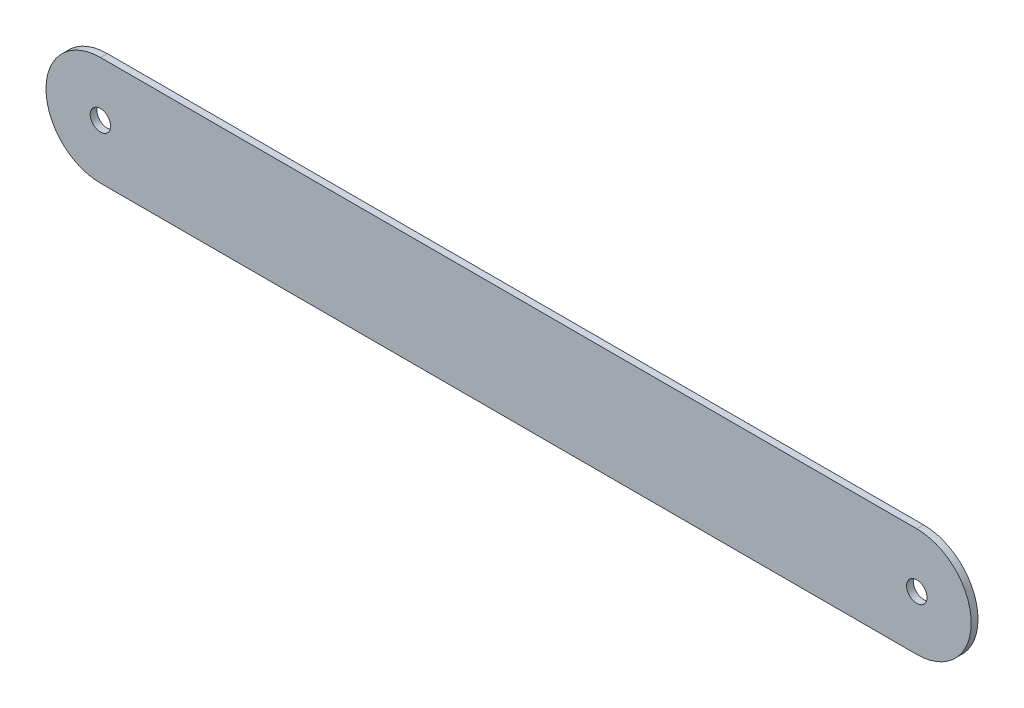
SolidWorks part; units mm, degrees
ref_plane "前视基准面" through (0, 0, 0) normal (0, 0, 1) x (1, 0, 0)
ref_plane "上视基准面" through (0, 0, 0) normal (0, 1, 0) x (1, 0, 0)
ref_plane "右视基准面" through (0, 0, 0) normal (1, 0, 0) x (0, 0, -1)
sketch "草图1" plane through (0, 0, 0) normal (0, 0, 1) x (1, 0, 0)
  line L0 (0, 0) -> (600, 0) construction
  line L1 (0, 40) -> (600, 40)
  line L2 (0, -40) -> (600, -40)
  arc A0 (0, 40) -> (0, -40) centre (0, 0) ccw
  arc A1 (600, -40) -> (600, 40) centre (600, 0) ccw
  point P3 (300, 0)
  dimension "D2" = 40
  dimension "D1" = 600
extrude "凸台-拉伸1" add sketch "草图1" along normal blind 5
sketch "草图2" plane through (0, 0, 5) normal (0, 0, 1) x (1, 0, 0)
  circle A0 centre (0, 0) radius 7.5
  circle A1 centre (600, 0) radius 7.5
  dimension "D1" = 15
extrude "切除-拉伸1" cut sketch "草图2" against normal through all
